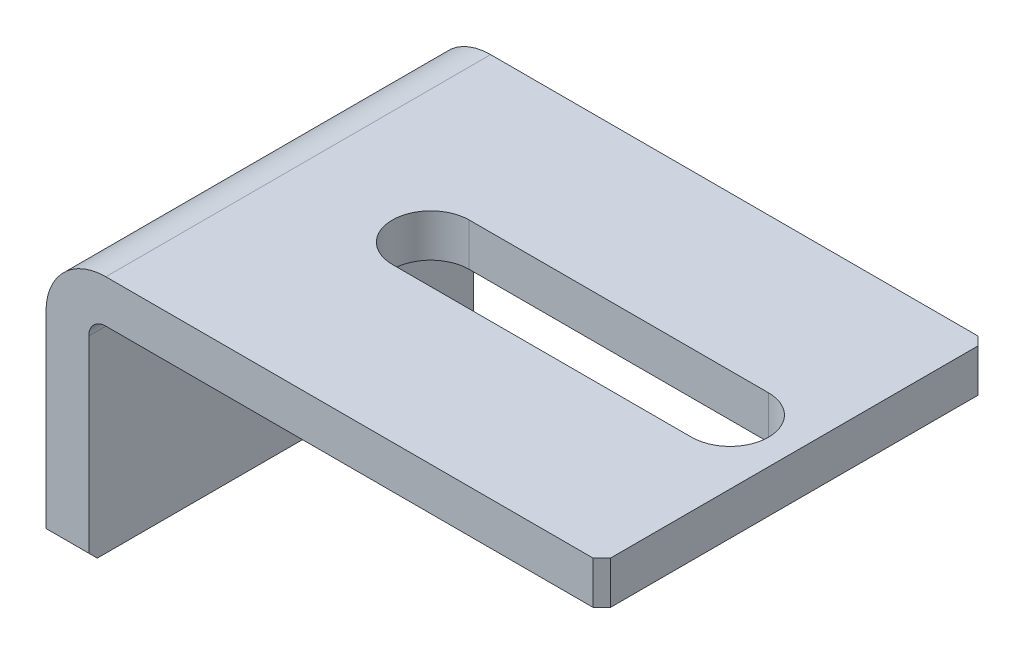
from build123d import *

# Parameters (mm, degrees)
EXTRUDE_1_DEPTH     = 45
FILLET_1_R          = 2
FILLET_2_R          = 7
CHAMFER_1_SIZE      = 1
CUT_EXTRUDE_1_DEPTH = 85.557672626


with BuildPart() as part:
    # 草图1 → 拉伸-薄壁1 (new body)
    with BuildSketch(Plane.XY):
        Polygon((0, 0), (0, 30), (65, 30), (65, 25), (5, 25), (5, 0), align=None)
    extrude(amount=EXTRUDE_1_DEPTH)

    # 圆角1
    fillet_1_edges = [part.edges().sort_by_distance(p)[0] for p in [
        (5, 25, 22.5),
    ]]
    fillet(fillet_1_edges, radius=FILLET_1_R)

    # 圆角2
    fillet_2_edges = [part.edges().sort_by_distance(p)[0] for p in [
        (0, 30, 22.5),
    ]]
    fillet(fillet_2_edges, radius=FILLET_2_R)

    # 倒角1
    chamfer_1_edges = [part.edges().sort_by_distance(p)[0] for p in [
        (2.5, 0, 45),
        (2.5, 0, 0),
        (65, 27.5, 0),
        (65, 27.5, 45),
    ]]
    chamfer(chamfer_1_edges, length=CHAMFER_1_SIZE)

    # 草图2 → 切除-拉伸1 (cut, through all)
    with BuildSketch(Plane(origin=(0, 30, 0), x_dir=(1, 0, 0), z_dir=(0, 1, 0))):
        with BuildLine():
            Line((22.5, -18), (57.5, -18))
            ThreePointArc((57.5, -18), (62, -22.5), (57.5, -27))
            Line((57.5, -27), (22.5, -27))
            ThreePointArc((22.5, -27), (18, -22.5), (22.5, -18))
        make_face()
    extrude(amount=-CUT_EXTRUDE_1_DEPTH, mode=Mode.SUBTRACT)


solid = part.part
